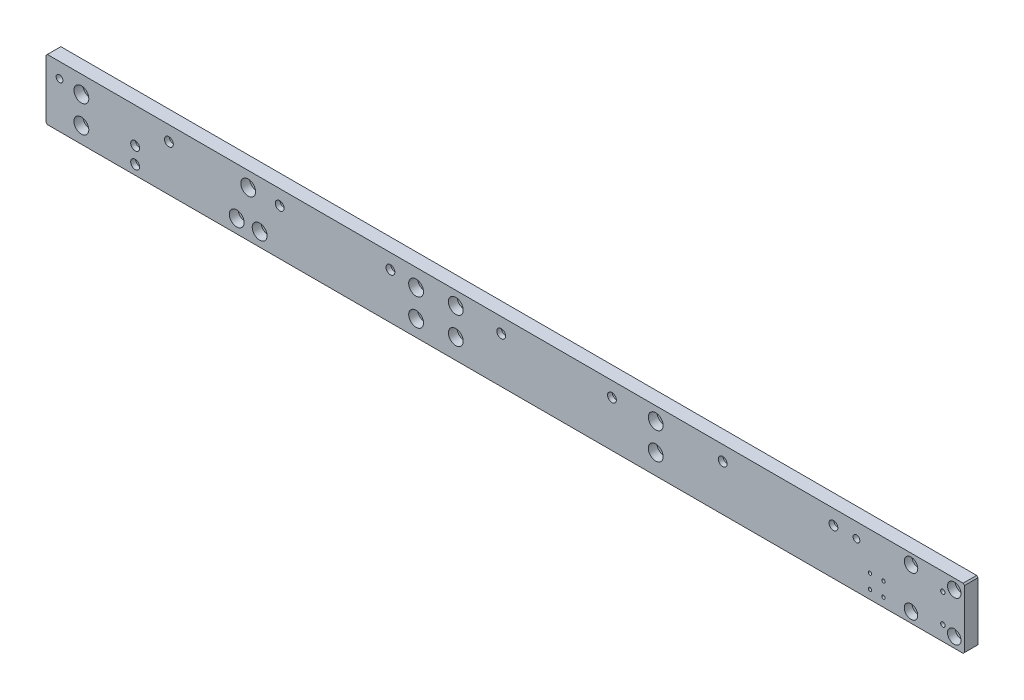
from build123d import *

# Parameters (mm, degrees)
SKETCH_1_W                    = 710
SKETCH_1_H                    = 45
EXTRUDE_1_DEPTH               = 10
HOLE_WIZARD_C_2_D             = 6.5
HOLE_WIZARD_C_2_CBORE_D       = 11
HOLE_WIZARD_C_2_CBORE_DEPTH   = 6.5
PATTERN_LINEAR_1_COUNT        = 7
PATTERN_LINEAR_1_PITCH        = 82
HOLE_WIZARD_C_1_D             = 6.6
HOLE_WIZARD_C_1_CBORE_D       = 11
HOLE_WIZARD_C_1_CBORE_DEPTH   = 6.6
HOLE_WIZARD_C_2_2_D           = 6.6
HOLE_WIZARD_C_2_2_CBORE_D     = 11
HOLE_WIZARD_C_2_2_CBORE_DEPTH = 6.6
HOLE_WIZARD_C_3_D             = 6.5
HOLE_WIZARD_C_3_CBORE_D       = 11
HOLE_WIZARD_C_3_CBORE_DEPTH   = 6.5
HOLE_WIZARD_M6_1_D            = 6.6
HOLE_WIZARD_M6_1_CBORE_D      = 11
HOLE_WIZARD_M6_1_CBORE_DEPTH  = 6.4
HOLE_WIZARD_M6_2_D            = 6.6
HOLE_WIZARD_M6_2_CBORE_D      = 11
HOLE_WIZARD_M6_2_CBORE_DEPTH  = 6.4
CHAMFER_1_SIZE                = 1
HOLE_WIZARD_5_0_5_1_D         = 5
HOLE_WIZARD_5_0_5_1_DEPTH     = 15.61
HOLE_WIZARD_5_0_5_1_TIP       = 1.443375673
HOLE_WIZARD_1_D               = 5.3
HOLE_WIZARD_1_CBORE_D         = 10
HOLE_WIZARD_1_CBORE_DEPTH     = 5.7
HOLE_WIZARD_M4_1_D            = 3.3
HOLE_WIZARD_M4_1_DEPTH        = 10.1
HOLE_WIZARD_M4_1_TIP          = 0.991420021
CUT_EXTRUDE_1_DEPTH           = 402.103477921
CUT_EXTRUDE_1_DEPTH_BACK      = 402.103477921
CHAMFER_2_SIZE                = 1
HOLE_WIZARD_M3_1_D            = 2.5
HOLE_WIZARD_M3_1_DEPTH        = 7.5
HOLE_WIZARD_M3_1_TIP          = 0.751075774


with BuildPart() as part:
    # 草图1 → 凸台-拉伸1 (new body)
    with BuildSketch(Plane.XY):
        with Locations((-45, -5.5)):
            Rectangle(SKETCH_1_W, SKETCH_1_H)
    extrude(amount=-EXTRUDE_1_DEPTH)

    # Hole Wizard C _2 (through all)
    with Locations(Plane(origin=(0, 0, -10), x_dir=(-1, 0, 0), z_dir=(0, 0, -1))):
        with Locations((-213, 6)):
            hole_wizard_c_2 = CounterBoreHole(HOLE_WIZARD_C_2_D / 2, HOLE_WIZARD_C_2_CBORE_D / 2, HOLE_WIZARD_C_2_CBORE_DEPTH)

    # 阵列(线性)1: Hole Wizard C _2 ×7
    with Locations(*[(-i * PATTERN_LINEAR_1_PITCH, 0, 0) for i in range(1, PATTERN_LINEAR_1_COUNT)]):
        add(hole_wizard_c_2, mode=Mode.SUBTRACT)

    # 打孔尺寸根据六角头螺栓 C 级的类型1 (through all)
    with Locations(Plane.XY):
        with Locations((-343.82, -16), (-343.82, 4)):
            CounterBoreHole(HOLE_WIZARD_C_1_D / 2, HOLE_WIZARD_C_1_CBORE_D / 2, HOLE_WIZARD_C_1_CBORE_DEPTH)

    # Hole Wizard C _2 2 (through all)
    with Locations(Plane.XY):
        with Locations((-96, -16), (-96, 4)):
            CounterBoreHole(HOLE_WIZARD_C_2_2_D / 2, HOLE_WIZARD_C_2_2_CBORE_D / 2, HOLE_WIZARD_C_2_2_CBORE_DEPTH)

    # 打孔尺寸根据六角头螺栓 C 级的类型3 (through all)
    with Locations(Plane.XY):
        with Locations((-228.82, -18), (-211.82, -18), (-220.32, 6)):
            CounterBoreHole(HOLE_WIZARD_C_3_D / 2, HOLE_WIZARD_C_3_CBORE_D / 2, HOLE_WIZARD_C_3_CBORE_DEPTH)

    # M6 六角凹头螺钉的柱形沉头孔1 (through all)
    with Locations(Plane(origin=(0, 0, -10), x_dir=(-1, 0, 0), z_dir=(0, 0, -1))):
        with Locations((304, -21), (304, -9)):
            CounterBoreHole(HOLE_WIZARD_M6_1_D / 2, HOLE_WIZARD_M6_1_CBORE_D / 2, HOLE_WIZARD_M6_1_CBORE_DEPTH)

    # M6 六角凹头螺钉的柱形沉头孔2 (through all)
    with Locations(Plane.XY):
        with Locations((81.400029989, 7), (81.400029989, -13), (-66.599970011, 7), (-66.599970011, -13)):
            CounterBoreHole(HOLE_WIZARD_M6_2_D / 2, HOLE_WIZARD_M6_2_CBORE_D / 2, HOLE_WIZARD_M6_2_CBORE_DEPTH)

    # 倒角1
    chamfer_1_edges = [part.edges().sort_by_distance(p)[0] for p in [
        (-400, 17, -5),
        (310, 17, -5),
        (310, -28, -5),
        (-400, -28, -5),
    ]]
    chamfer(chamfer_1_edges, length=CHAMFER_1_SIZE)

    # Ø5.0 (5) 直径孔1
    with Locations(Plane.XY):
        with Locations((230, 6), (-360, 6)):
            Hole(HOLE_WIZARD_5_0_5_1_D / 2, depth=HOLE_WIZARD_5_0_5_1_DEPTH)
            with Locations((0, 0, -(HOLE_WIZARD_5_0_5_1_DEPTH + HOLE_WIZARD_5_0_5_1_TIP / 2))):  # 120° drill point
                Cone(0, HOLE_WIZARD_5_0_5_1_D / 2, HOLE_WIZARD_5_0_5_1_TIP, mode=Mode.SUBTRACT)

    # 打孔尺寸根据内六角圆柱头螺钉的类型1 (through all)
    with Locations(Plane.XY):
        with Locations((270.4, 9.5), (302.4, 9.5), (270.4, -20.5), (302.4, -20.5)):
            CounterBoreHole(HOLE_WIZARD_1_D / 2, HOLE_WIZARD_1_CBORE_D / 2, HOLE_WIZARD_1_CBORE_DEPTH)

    # M4 螺纹孔1
    with Locations(Plane.XY):
        with Locations((294, 4), (294, -17)):
            Hole(HOLE_WIZARD_M4_1_D / 2, depth=HOLE_WIZARD_M4_1_DEPTH)
            with Locations((0, 0, -(HOLE_WIZARD_M4_1_DEPTH + HOLE_WIZARD_M4_1_TIP / 2))):  # 118° drill point
                Cone(0, HOLE_WIZARD_M4_1_D / 2, HOLE_WIZARD_M4_1_TIP, mode=Mode.SUBTRACT)

    # 草图21 → 切除-拉伸1 (cut, two sides: drawn at the far end of the back side and taken through both)
    with BuildSketch(Plane.XY.offset(-CUT_EXTRUDE_1_DEPTH_BACK)):
        Polygon((-370, 1426.732120581), (-370, 48.216256267), (-370, -32.871094122), (-370, -1411.386958436), (-3127.031728627, -1411.386958436), (-3127.031728627, 1426.732120581), align=None)
    extrude(amount=CUT_EXTRUDE_1_DEPTH + CUT_EXTRUDE_1_DEPTH_BACK, mode=Mode.SUBTRACT)

    # 倒角2
    chamfer_2_edges = [part.edges().sort_by_distance(p)[0] for p in [
        (-370, -28, -5),
        (-370, 17, -5),
    ]]
    chamfer(chamfer_2_edges, length=CHAMFER_2_SIZE)

    # M3 螺纹孔1
    with Locations(Plane.XY):
        with Locations((240, -21.5), (240, -11.1), (250, -11.1), (250, -21.5)):
            Hole(HOLE_WIZARD_M3_1_D / 2, depth=HOLE_WIZARD_M3_1_DEPTH)
            with Locations((0, 0, -(HOLE_WIZARD_M3_1_DEPTH + HOLE_WIZARD_M3_1_TIP / 2))):  # 118° drill point
                Cone(0, HOLE_WIZARD_M3_1_D / 2, HOLE_WIZARD_M3_1_TIP, mode=Mode.SUBTRACT)


solid = part.part
